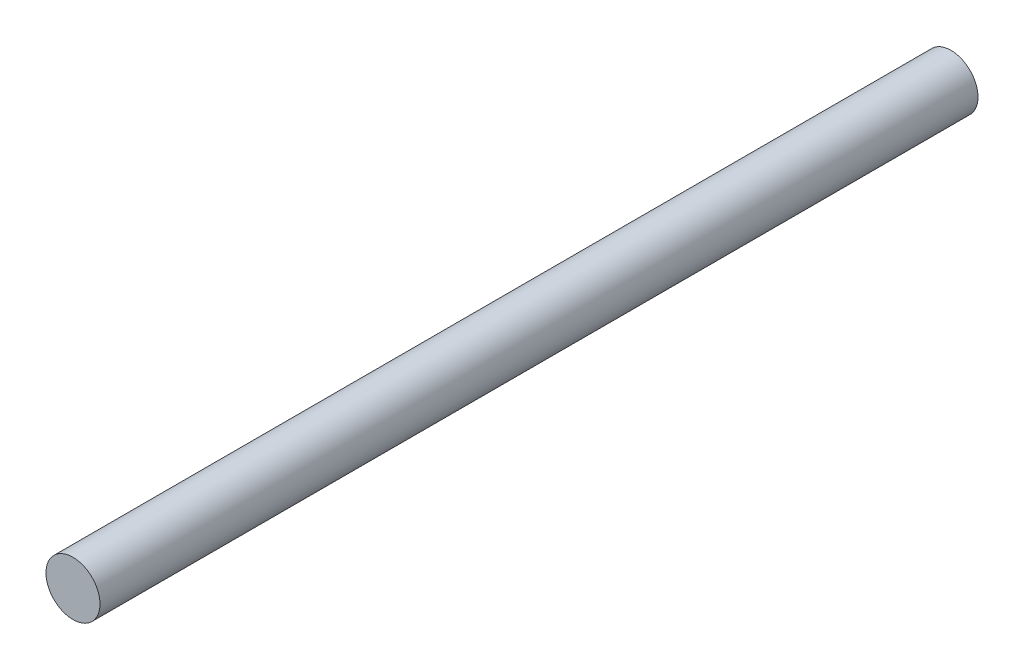
SolidWorks part; units mm, degrees
ref_plane "Front Plane" through (0, 0, 0) normal (0, 0, 1) x (1, 0, 0)
ref_plane "Top Plane" through (0, 0, 0) normal (0, 1, 0) x (1, 0, 0)
ref_plane "Right Plane" through (0, 0, 0) normal (1, 0, 0) x (0, 0, -1)
other "Configuration Table"
sketch "Sketch1" plane through (0, 0, 0) normal (0, 0, 1) x (1, 0, 0)
  circle A0 centre (162.9385, 320.2262) radius 4
  circle A1 centre (203.4606, 349.1309) radius 4
  circle A2 centre (233.3705, 361.8006) radius 4
extrude "Boss-Extrude1" add sketch "Sketch1" against normal up to surface (130 mm away) contours A2
